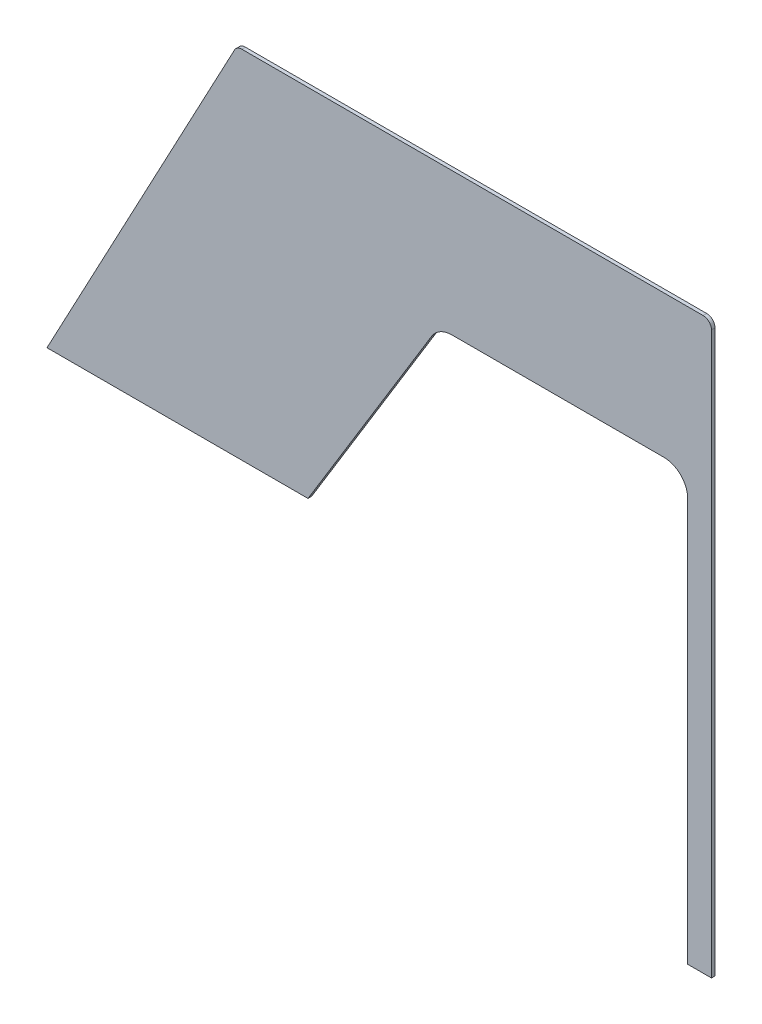
from build123d import *

# Parameters (mm, degrees)
BOSS_EXTRUDE1_DEPTH = 1.5


with BuildPart() as part:
    # Sketch1 → Boss-Extrude1 (new body)
    with BuildSketch(Plane.XY):
        with BuildLine():
            Line((0, 0), (79.011764706, 148.147058824))
            ThreePointArc((79.011764706, 148.147058824), (80.299264856, 149.50122524), (82.1, 150))
            Line((82.1, 150), (276.5, 150))
            ThreePointArc((276.5, 150), (278.974873734, 148.974873734), (280, 146.5))
            Line((280, 146.5), (280, -90))
            Line((280, -90), (270, -90))
            Line((270, -90), (270, 80))
            ThreePointArc((270, 80), (267.071067812, 87.071067812), (260, 90))
            Line((260, 90), (170.608346172, 90))
            ThreePointArc((170.608346172, 90), (165.716771832, 88.721955083), (162.075527836, 85.214500095))
            Line((162.075527836, 85.214500095), (110, 0))
            Line((110, 0), (0, 0))
        make_face()
    extrude(amount=BOSS_EXTRUDE1_DEPTH)


solid = part.part
